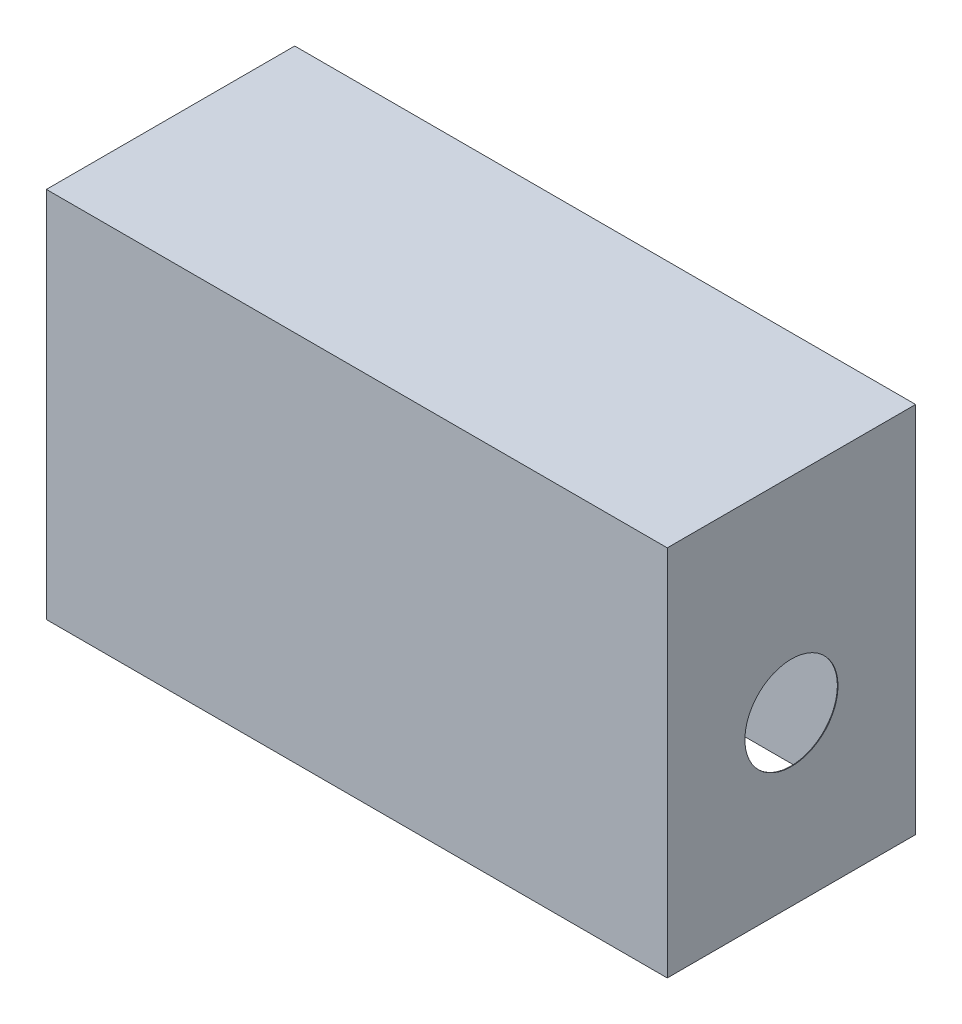
from build123d import *

# Parameters (mm, degrees)
SKETCH1_W           = 1000
SKETCH1_H           = 400
BOSS_EXTRUDE1_DEPTH = 600
SKETCH2_W           = 998
SKETCH2_H           = 398
CUT_EXTRUDE1_DEPTH  = 599
SKETCH3_R           = 75
CUT_EXTRUDE2_DEPTH  = 50


with BuildPart() as part:
    # Sketch1 → Boss-Extrude1 (new body)
    with BuildSketch(Plane(origin=(0, 0, 0), x_dir=(1, 0, 0), z_dir=(0, 1, 0))):
        Rectangle(SKETCH1_W, SKETCH1_H)
    extrude(amount=BOSS_EXTRUDE1_DEPTH)

    # Sketch2 → Cut-Extrude1 (cut)
    with BuildSketch(Plane.XZ):
        Rectangle(SKETCH2_W, SKETCH2_H)
    extrude(amount=-CUT_EXTRUDE1_DEPTH, mode=Mode.SUBTRACT)

    # Sketch3 → Cut-Extrude2 (cut)
    with BuildSketch(Plane(origin=(500, 0, 0), x_dir=(0, 0, -1), z_dir=(1, 0, 0))):
        with Locations((0, 270)):
            Circle(SKETCH3_R)
    extrude(amount=-CUT_EXTRUDE2_DEPTH, mode=Mode.SUBTRACT)


solid = part.part
